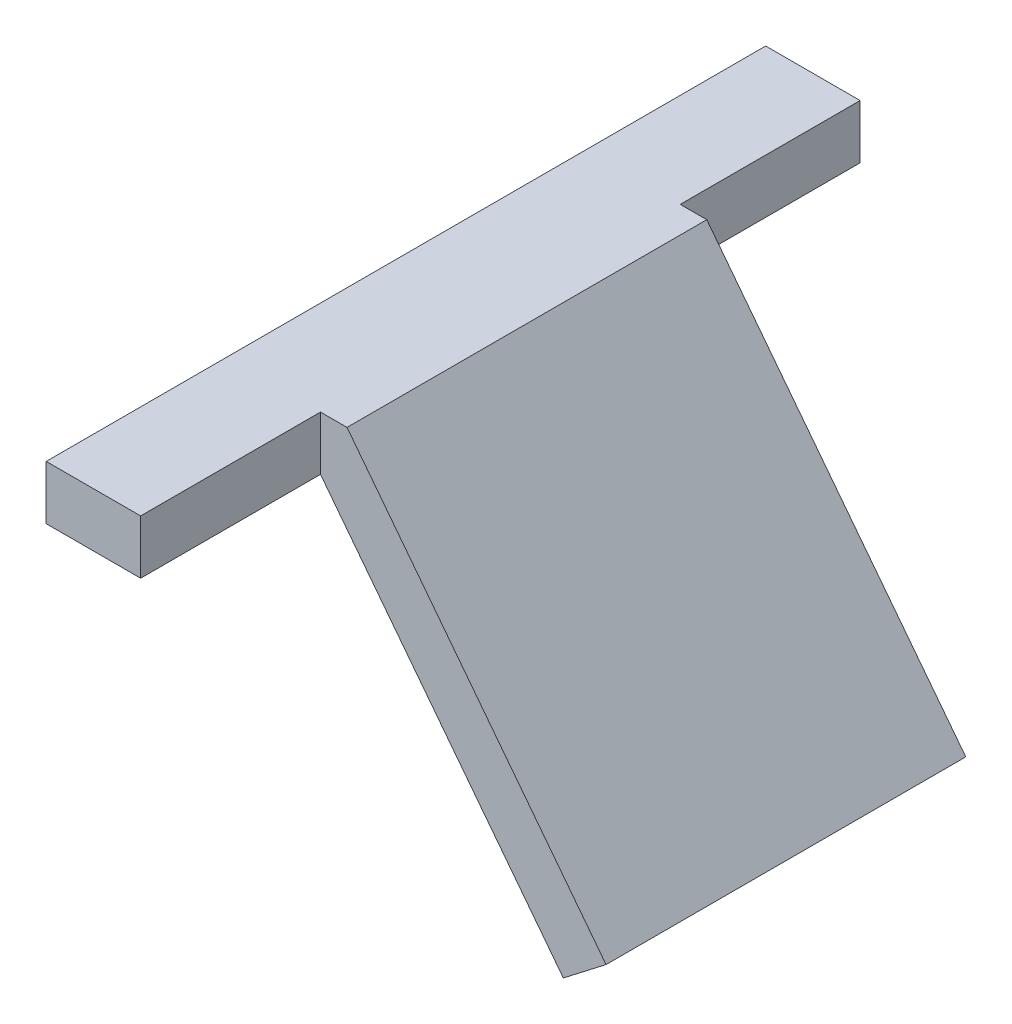
from build123d import *

# Parameters (mm, degrees)
BOSS_EXTRUDE2_DEPTH = 20
SKETCH4_W           = 10.5
SKETCH4_H           = 6
BOSS_EXTRUDE3_DEPTH = 20


with BuildPart() as part:
    # Sketch3 → Boss-Extrude2 (new, symmetric)
    with BuildSketch(Plane.XY):
        Polygon((0, 0), (10.5, 0), (37.498965991, -34.995654522), (42.249507329, -31.330636514), (13.449114839, 6), (0, 6), align=None)
    extrude(amount=BOSS_EXTRUDE2_DEPTH, both=True)

    # Sketch4 → Boss-Extrude3 (add)
    with BuildSketch(Plane.XY.offset(20)):
        with Locations((5.25, 3)):
            Rectangle(SKETCH4_W, SKETCH4_H)
    boss_extrude3 = extrude(amount=BOSS_EXTRUDE3_DEPTH)

    # Mirror1: Boss-Extrude3 across plane
    add(boss_extrude3.mirror(Plane.XY))


solid = part.part
